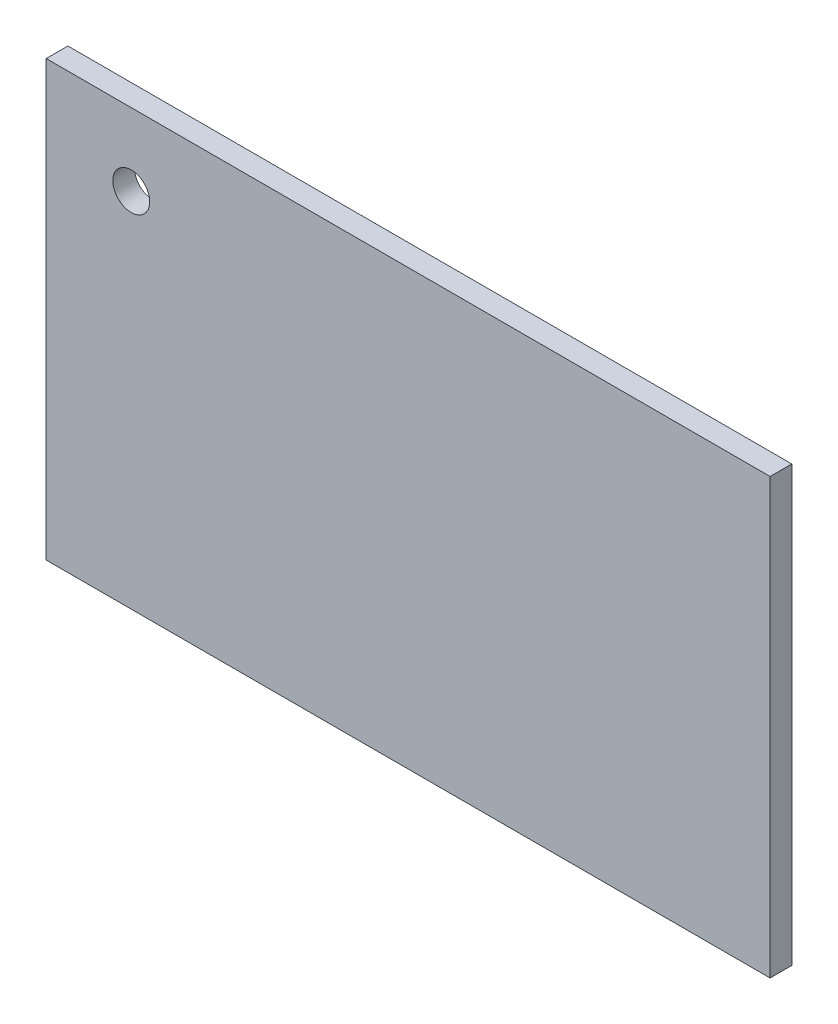
from build123d import *

# Parameters (mm, degrees)
SKETCH1_W              = 200
SKETCH1_H              = 120
BOSS_EXTRUDE1_DEPTH    = 6
M12_TAPPED_HOLE1_D     = 10.2
M12_TAPPED_HOLE1_DEPTH = 29.25
M12_TAPPED_HOLE1_TIP   = 3.064389157


with BuildPart() as part:
    # Sketch1 → Boss-Extrude1 (new body)
    with BuildSketch(Plane.XY):
        Rectangle(SKETCH1_W, SKETCH1_H)
    extrude(amount=BOSS_EXTRUDE1_DEPTH)

    # M12 Tapped Hole1
    with Locations(Plane.XY.offset(6)):
        with Locations((-76.5, 40)):
            Hole(M12_TAPPED_HOLE1_D / 2, depth=M12_TAPPED_HOLE1_DEPTH)
            with Locations((0, 0, -(M12_TAPPED_HOLE1_DEPTH + M12_TAPPED_HOLE1_TIP / 2))):  # 118° drill point
                Cone(0, M12_TAPPED_HOLE1_D / 2, M12_TAPPED_HOLE1_TIP, mode=Mode.SUBTRACT)


solid = part.part
